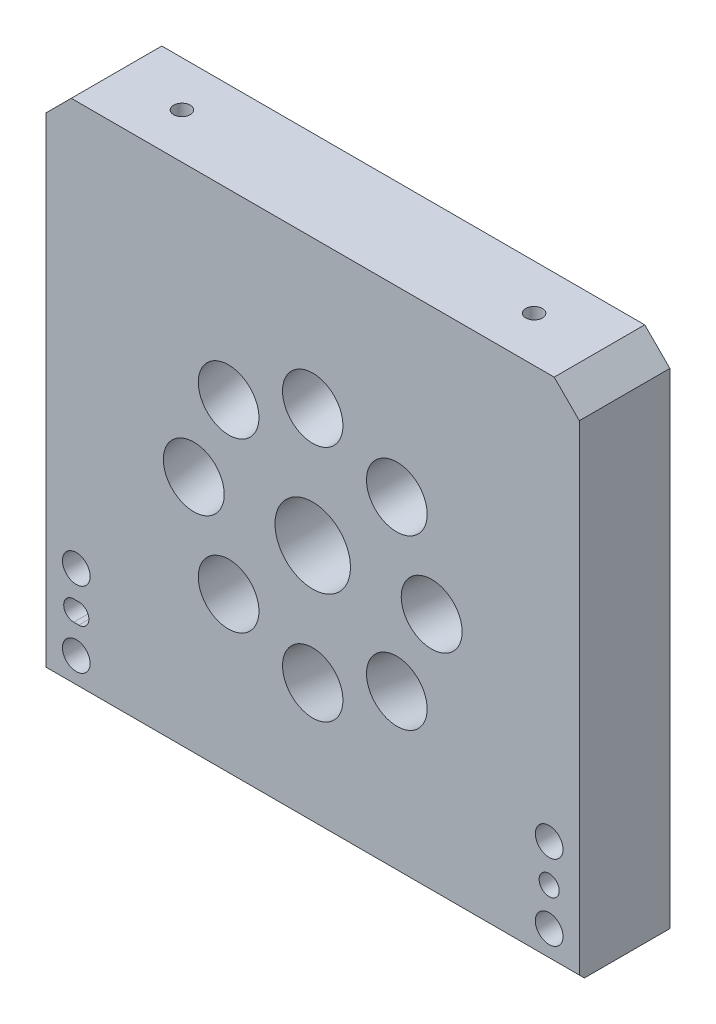
from build123d import *

# Parameters (mm, degrees)
SKETCH1_W                                            = 106
SKETCH1_H                                            = 101.44
BOSS_EXTRUDE1_DEPTH                                  = 9
SKETCH3_R                                            = 7.5
CUT_EXTRUDE1_DEPTH                                   = 76.534882008
CIRPATTERN1_COUNT                                    = 8
CHAMFER1_SIZE                                        = 5
CHAMFER2_SIZE                                        = 1
HOLE_SIZE_PER_SOCKET_HEAD_CAP_SCREW_TYPE_D           = 5.5
HOLE_SIZE_PER_SOCKET_HEAD_CAP_SCREW_TYPE_CBORE_D     = 9.5
HOLE_SIZE_PER_SOCKET_HEAD_CAP_SCREW_TYPE_CBORE_DEPTH = 6
M4_TAPPED_HOLE1_D                                    = 3.3
M4_TAPPED_HOLE1_DEPTH                                = 12.1
M4_TAPPED_HOLE1_TIP                                  = 0.991420021
SKETCH11_R                                           = 2
CUT_EXTRUDE2_DEPTH                                   = 76.534882008


with BuildPart() as part:
    # Sketch1 → Boss-Extrude1 (new, symmetric)
    with BuildSketch(Plane.XY):
        Rectangle(SKETCH1_W, SKETCH1_H)
    extrude(amount=BOSS_EXTRUDE1_DEPTH, both=True)

    # Sketch3 → Cut-Extrude1 (cut, through all)
    with BuildSketch(Plane(origin=(0, 0, -9), x_dir=(-1, 0, 0), z_dir=(0, 0, -1))):
        with Locations((0, -2.277412343)):
            Circle(SKETCH3_R)
    extrude(amount=-CUT_EXTRUDE1_DEPTH, mode=Mode.SUBTRACT)

    # Sketch2 → Cut-Revolve1 (revolve, cut)
    with BuildSketch(Plane(origin=(0, 0, 0), x_dir=(0, 0, -1), z_dir=(1, 0, 0)), mode=Mode.PRIVATE) as cut_revolve1_sk:
        Polygon((6.863117782, 17.401707924), (7.124170166, 15.418818201), (16.047173919, 16.593553931), (15.002964381, 24.525112822), (-9.783157153, 21.261958017), (-9, 15.313288849), align=None)
    cut_revolve1 = revolve(cut_revolve1_sk.sketch.rotate(Axis((0, 24.525112822, -15.002964381), (0, -0.1305261922200479, 0.9914448613738109)), 180), axis=Axis((0, 24.525112822, -15.002964381), (0, -0.1305261922200479, 0.9914448613738109)), mode=Mode.SUBTRACT)

    # Sketch4 → M3 Tapped Hole1 (revolve, cut)
    with BuildSketch(Plane(origin=(0, 9.166817967, -9), x_dir=(0, 1, 0), z_dir=(1, 0, 0))):
        Polygon((0, 0), (0, 8.251075774), (1.25, 7.5), (1.25, 0), align=None)
    m3_tapped_hole1 = revolve(axis=Axis((0, 9.166817967, -15.35), (0, 0, 1)), mode=Mode.SUBTRACT)

    # CirPattern1: Cut-Revolve1, M3 Tapped Hole1 ×8 about axis
    cirpattern1_axis = Axis((0, -2.277412343, 0), (0, 0, 1))
    add([cut_revolve1.rotate(cirpattern1_axis, i * 360 / CIRPATTERN1_COUNT) for i in range(1, CIRPATTERN1_COUNT)], mode=Mode.SUBTRACT)
    add([m3_tapped_hole1.rotate(cirpattern1_axis, i * 360 / CIRPATTERN1_COUNT) for i in range(1, CIRPATTERN1_COUNT)], mode=Mode.SUBTRACT)

    # Chamfer1
    chamfer1_edges = [part.edges().sort_by_distance(p)[0] for p in [
        (-53, 50.72, 0),
        (53, 50.72, 0),
    ]]
    chamfer(chamfer1_edges, length=CHAMFER1_SIZE)

    # Chamfer2
    chamfer2_edges = [part.edges().sort_by_distance(p)[0] for p in [
        (0, -50.72, 9),
    ]]
    chamfer(chamfer2_edges, length=CHAMFER2_SIZE)

    # Hole size per socket head cap screw type1 (through all)
    with Locations(Plane(origin=(0, 0, -9), x_dir=(-1, 0, 0), z_dir=(0, 0, -1))):
        with Locations((-47, -29.72), (-47, -44.72), (47, -44.72), (47, -29.72)):
            CounterBoreHole(HOLE_SIZE_PER_SOCKET_HEAD_CAP_SCREW_TYPE_D / 2, HOLE_SIZE_PER_SOCKET_HEAD_CAP_SCREW_TYPE_CBORE_D / 2, HOLE_SIZE_PER_SOCKET_HEAD_CAP_SCREW_TYPE_CBORE_DEPTH)

    # M4 Tapped Hole1
    with Locations(Plane(origin=(0, 50.72, 0), x_dir=(1, 0, 0), z_dir=(0, 1, 0))):
        with Locations((-35, 0), (35, 0)):
            Hole(M4_TAPPED_HOLE1_D / 2, depth=M4_TAPPED_HOLE1_DEPTH)
            with Locations((0, 0, -(M4_TAPPED_HOLE1_DEPTH + M4_TAPPED_HOLE1_TIP / 2))):  # 118° drill point
                Cone(0, M4_TAPPED_HOLE1_D / 2, M4_TAPPED_HOLE1_TIP, mode=Mode.SUBTRACT)

    # Sketch11 → Cut-Extrude2 (cut, through all)
    with BuildSketch(Plane(origin=(0, 0, -9), x_dir=(-1, 0, 0), z_dir=(0, 0, -1))):
        with Locations((-47, -37.22)):
            Circle(SKETCH11_R)
        with BuildLine():
            Line((46.5, -35.22), (47.5, -35.22))
            ThreePointArc((47.5, -35.22), (49.5, -37.22), (47.5, -39.22))
            Line((47.5, -39.22), (46.5, -39.22))
            ThreePointArc((46.5, -39.22), (44.5, -37.22), (46.5, -35.22))
        make_face()
    extrude(amount=-CUT_EXTRUDE2_DEPTH, mode=Mode.SUBTRACT)


solid = part.part
